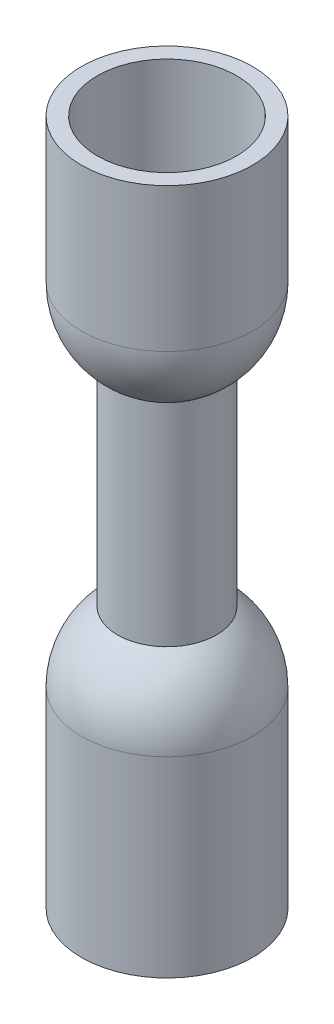
SolidWorks part; units mm, degrees
material "ABS"
ref_plane "Front Plane" through (0, 0, 0) normal (0, 0, 1) x (1, 0, 0)
ref_plane "Top Plane" through (0, 0, 0) normal (0, 1, 0) x (1, 0, 0)
ref_plane "Right Plane" through (0, 0, 0) normal (1, 0, 0) x (0, 0, -1)
sketch "Sketch1" plane through (0, 0, 0) normal (0, 0, 1) x (1, 0, 0)
  line L1 (-1.05, 15.0834) -> (-1.05, 7.9105)
  line L2 (-2.18, 16.9939) -> (-2.18, 21.4939)
  line L4 (-2.18, 6) -> (-2.18, 0)
  line L5 (0, 24.1723) -> (0, -3.143) construction
  arc A2 (-2.18, 16.9939) -> (-1.05, 15.0834) centre (0, 16.9939) ccw
  arc A3 (-1.05, 7.9105) -> (-2.18, 6) centre (0, 6) ccw
  dimension "D3" = 2.18
  dimension "D6" = 2.18
  dimension "D1" = 6
  dimension "D2" = 4.5
  dimension "D4" = 21.4939
  dimension "D5" = 7.1729
  dimension "D7" = 1.13
  dimension "D8" = 1.13
revolve "Revolve-Thin1" add sketch "Sketch1" angle 360 about L5
